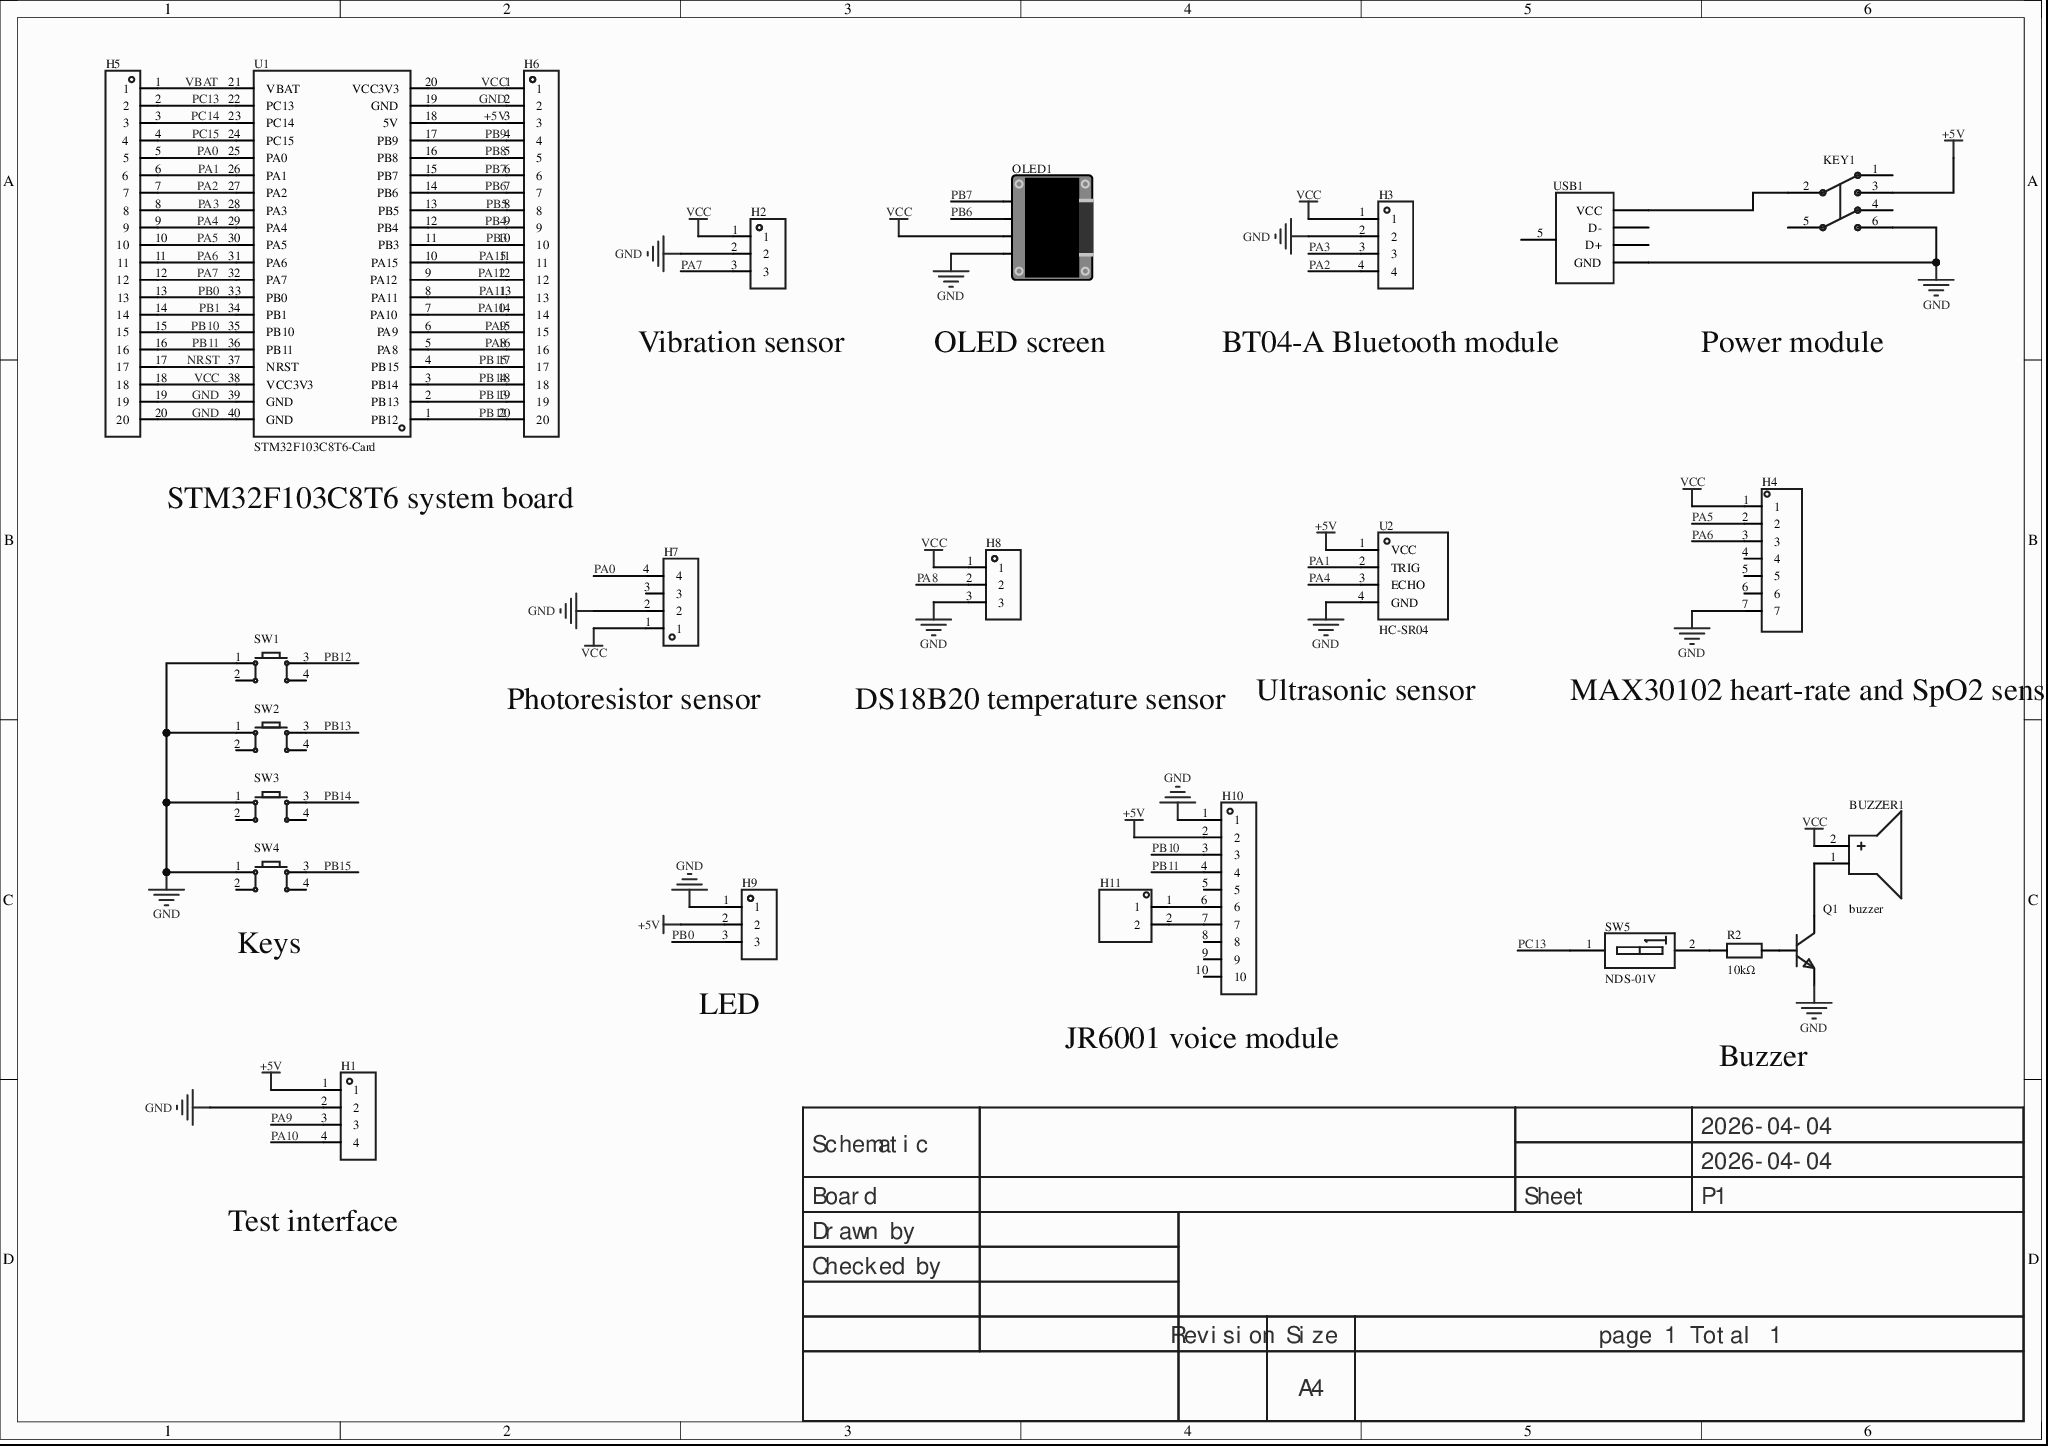
[diagram p0: MISC61230-3.schdoc]
# Altium project MISC61230-2.PrjPcb
1 sheet, 24 parts. Net scope: global (net labels, ports and power ports of the same name join across sheets).
Board file: MISC61230.pcbdoc

## Sheet MISC61230-3.schdoc
size 297 x 209 mm; Version: V1.0; @Project Name: MISC61230; @Page Count: 1; @Update Date: 2026-04-04; @Create Date: 2026-04-04; @Schematic Name: MISC61230; @Page No: 1; @Create Time: 18:58:15; @Update Time: 22:44:58; @Board Name: MISC61230

### Parts
BUZZER1  buzzer  [BUZ-TH_BD12.0-P6.00-D0.9-RD]
H1  (no value)  [HDR-TH_4P-P2.54-V-M]
H2  (no value)  [HDR-TH_3P-P2.54-V-F]
H3  (no value)  [HDR-TH_4P-P2.54-V-M]
H4  (no value)  [HDR-TH_7P-P2.54-V-F]
H5  (no value)  [HDR-TH_20P-P2.54-V-M-1]
H6  (no value)  [HDR-TH_20P-P2.54-V-M-1]
H7  (no value)  [HDR-TH_4P-P2.54-V-M]
H8  (no value)  [HDR-TH_3P-P2.54-V-F]
H9  (no value)  [HDR-TH_3P-P2.54-V-F]
H10  (no value)  [HDR-TH_10P-P2.54-V-F]
H11  (no value)  [HDR-TH_2P-P2.54-V-M-1]
KEY1  Non-latching switch 8.5×8.5, silent  [SW-TH_6P-L8.5-W8.5-P2.54]  (value not drawn)
OLED1  (no value)  [0.96OLED_4P]
Q1  (no value)  [S8050_TO_92]
R2  10kΩ  [Res_1/8W]
SW1  (no value)  [SW-TH_4P-L6.0-W6.0-P4.50-LS6.5]
SW2  (no value)  [SW-TH_4P-L6.0-W6.0-P4.50-LS6.5]
SW3  (no value)  [SW-TH_4P-L6.0-W6.0-P4.50-LS6.5]
SW4  (no value)  [SW-TH_4P-L6.0-W6.0-P4.50-LS6.5]
SW5  NDS-01V  [SW-TH_2P-L3.9-W9.9-P2.54-LS7.6]
U1  STM32F103C8T6-Card  [CONN-TH_L53.3-W22.9_STM32F103C8T6-CARD]
U2  HC-SR04  [TH_HC-SR04V]
USB1  (no value)  [USB_ Type-B]

### Nets
+5V: H1.1 H6.3 H9.2 H10.2 KEY1.3 U1.18(5V) U2.1(VCC)
GND: H1.2 H2.2 H3.2 H4.7 H5.19 H5.20 H6.2 H7.2 H8.3 H9.1 H10.1 KEY1.6 OLED1.1(GND) Q1.1(E) SW1.1 SW2.1 SW3.1 SW4.1 U1.19(GND) U1.39(GND) U1.40(GND) U2.4(GND) USB1.4(GND)
VCC: BUZZER1.2(+) H2.1 H3.1 H4.1 H5.18 H6.1 H7.1 H8.1 OLED1.2(VCC) U1.20(VCC3V3) U1.38(VCC3V3)
NRST: H5.17 U1.37(NRST)
PA0: H5.5 H7.4 U1.25(PA0)
PA1: H5.6 U1.26(PA1) U2.2(TRIG)
PA2: H3.4 H5.7 U1.27(PA2)
PA3: H3.3 H5.8 U1.28(PA3)
PA4: H5.9 U1.29(PA4) U2.3(ECHO)
PA5: H4.2 H5.10 U1.30(PA5)
PA6: H4.3 H5.11 U1.31(PA6)
PA7: H2.3 H5.12 U1.32(PA7)
PA8: H6.16 H8.2 U1.5(PA8)
PA9: H1.3 H6.15 U1.6(PA9)
PA10: H1.4 H6.14 U1.7(PA10)
PA11: H6.13 U1.8(PA11)
PA12: H6.12 U1.9(PA12)
PA15: H6.11 U1.10(PA15)
PB0: H5.13 H9.3 U1.33(PB0)
PB1: H5.14 U1.34(PB1)
PB3: H6.10 U1.11(PB3)
PB4: H6.9 U1.12(PB4)
PB5: H6.8 U1.13(PB5)
PB6: H6.7 OLED1.3(SCL) U1.14(PB6)
PB7: H6.6 OLED1.4(SDA) U1.15(PB7)
PB8: H6.5 U1.16(PB8)
PB9: H6.4 U1.17(PB9)
PB10: H5.15 H10.3 U1.35(PB10)
PB11: H5.16 H10.4 U1.36(PB11)
PB12: H6.20 SW1.3 U1.1(PB12)
PB13: H6.19 SW2.3 U1.2(PB13)
PB14: H6.18 SW3.3 U1.3(PB14)
PB15: H6.17 SW4.3 U1.4(PB15)
PC13: H5.2 SW5.1(A1) U1.22(PC13)
PC14: H5.3 U1.23(PC14)
PC15: H5.4 U1.24(PC15)
VBAT: H5.1 U1.21(VBAT)
NetBUZZER1_1: BUZZER1.1(-) Q1.3(C)
NetH10_6: H10.6 H11.1
NetH10_7: H10.7 H11.2
NetKEY1_2: KEY1.2 USB1.1(VCC)
NetQ1_2: Q1.2(B) R2.2
NetR2_1: R2.1 SW5.2(A2)

Not connected (* = marked no-connect by the designer): H4 4 5 6; H7 3; H10 5 8 9 10; KEY1 1 4 5; SW1 2 4; SW2 2 4; SW3 2 4; SW4 2 4; USB1 2(D-)* 3(D+)* 5(SH1)

### Notes on the sheet
- (near H2) Vibration sensor
- OLED screen
- BT04-A Bluetooth module
- Power module
- STM32F103C8T6 system board
- (near H7) Photoresistor sensor
- DS18B20 temperature sensor
- Ultrasonic sensor
- (near H4) MAX30102 heart-rate and SpO2 sensor
- (near SW4) Keys
- (near H9) LED
- (near H10) JR6001 voice module
- Buzzer
- (near H1) Test interface
- 2026-04-04
- Schematic
- Board
- Sheet
- P1
- Drawn by
- Checked by
- Revision
- Size
- A4
- page 1 Total 1

### Library data of the parts
BUZZER1 = buzzer: AddInBom: yes; ModelId: af17e4151ed84fc2a628230bf23763630819f05c4eef4c71ace90d822a990e87; ModelTransform: 472.44,472.176,0,270,0,0,0,0,-196.85; Symbol: BUZZER; Device: buzzer; LCSC Part Name: buzzer; SupplierPart: C9900014030; ManufacturerPart: buzzer; Supplier Footprint: buzzer; JLCPCB Part Class: Extended Part; Supplier: LCSC; ConvertToPcb: yes; FootprintName: BUZ-TH_BD12.0-P6.00-D0.9-RD; ModelName: BUZ-TH_BD12.0-P6.00-D0.9-RD
H1 = HDR-M_2.54_1x4P: Symbol: PZ254V-11-04P; ConvertToPcb: yes; ModelId: 112f4d05e8d64e99ab9a333894bea4f90819f05c4eef4c71ace90d822a990e87; ModelName: HDR-TH_4P-P2.54-M-LI-1X4P; ModelTransform: 399.999,104.7242,0,0,0,0,0,0,-118.11; Device: HDR-M_2.54_1x4P; AddInBom: yes; SupplierPart: C492403; Supplier Footprint: 插件; FootprintName: HDR-TH_4P-P2.54-V-M
H2 H8 H9 = HDR-F_2.54_1x3P: Symbol: PM254V-11-03-H85; 3D Model: f3b3cc5aae9641bf9e56fc160cef875b; 3D Model Transform: 299.9994,100,0,0,0,0,0,0,-118.11; ConvertToPcb: yes; ModelName: HDR2.54-F-LI-1X3P; Device: HDR-F_2.54_1x3P; Supplier Part: C541850; Supplier Footprint: 插件; AddInBom: yes; FootprintName: HDR-TH_3P-P2.54-V-F
H3 H7 = HDR-M_2.54_1x4P: Symbol: PZ254V-11-04P; 3D Model: 112f4d05e8d64e99ab9a333894bea4f90819f05c4eef4c71ace90d822a990e87; 3D Model Transform: 399.999,104.7242,0,0,0,0,0,0,-118.11; ConvertToPcb: yes; ModelName: HDR-TH_4P-P2.54-M-LI-1X4P; Device: HDR-M_2.54_1x4P; Supplier Part: C492403; Supplier Footprint: 插件; AddInBom: yes; FootprintName: HDR-TH_4P-P2.54-V-M
H4 = HDR-F_2.54_1x7P: Symbol: 220S-1*7P H=8.5MM Ytype Gold-plated; ConvertToPcb: yes; ModelId: 4c31987253bc43b9b52c17be2a6d3f910819f05c4eef4c71ace90d822a990e87; ModelName: HDR-TH_7P-P2.54-F-LI-1X7P; ModelTransform: 715.7466,94.488,0,0,0,0,0,0,-118.11; Device: HDR-F_2.54_1x7P; AddInBom: yes; SupplierPart: C124418; Supplier Footprint: 插件; FootprintName: HDR-TH_7P-P2.54-V-F
H5 H6 = HDR-M_2.54_1x20P: Pitch:2.54mm;total pins:20;rows:1;pin structure:-;row spacing:-;mounting type:through-hole;round/square pin:-;rated current:-;rated voltage:-;mating pin length:-;plastic height:-;contact material:brass;contact plating:-;colour:black;; Symbol: HDR_2.54-1x20P; ConvertToPcb: yes; ModelId: f68709be121d406db68b06f32a5953890819f05c4eef4c71ace90d822a990e87; ModelName: HDR-M-2.54_1x20; ModelTransform: 1999.996,100,0,0,0,0,0,0,-118.11; Device: HDR-M_2.54_1x20P; AddInBom: yes; SupplierPart: C50981; Supplier Footprint: 插件; FootprintName: HDR-TH_20P-P2.54-V-M-1
H10 = HDR-F_2.54_1x10P: Symbol: X5511FV-10-C70D30-1000; AddInBom: yes; ModelId: 08a5ee31ec6747838a696d2ac093ffa40819f05c4eef4c71ace90d822a990e87; ModelName: HDR-TH_10P-P2.54-F-LI-1X10P; ModelTransform: 1009.87987,100,0,0,0,0,0,0,-125.984; Device: HDR-F_2.54_1x10P; ConvertToPcb: yes; FootprintName: HDR-TH_10P-P2.54-V-F; SupplierPart: C2684744; Supplier Footprint: 插件
H11 = HDR-M_2.54_1x2P: Symbol: 210S-1*2P L=11.6MMGold-plated black; ConvertToPcb: yes; ModelId: 79b2e9f2d70a4d68a1b7098f27c6d4c50819f05c4eef4c71ace90d822a990e87; ModelName: HDR-M-2.54_1x2; ModelTransform: 200,100,0,0,0,0,0,0,-118.11; Device: HDR-M_2.54_1x2P; AddInBom: yes; SupplierPart: C124375; Supplier Footprint: 插件; FootprintName: HDR-TH_2P-P2.54-V-M-1
KEY1 = 无自锁开关 8.5×8.5 无声: 6-pin, 8.5×8.5; Symbol: No self-locking switch 8.5×8.5 silent; AddInBom: yes; ModelId: 4c72b3966b92446eb355e1bd0fb4f8800819f05c4eef4c71ace90d822a990e87; ModelTransform: 342.519,334.645,0,180,0,0,0,0,-137.795; Device: Non-latching switch 8.5×8.5, silent; LCSC Part Name: 无自锁开关 8.5×8.5  无声; SupplierPart: C26228; ManufacturerPart: 无自锁开关 8.5×8.5 无声; Supplier Footprint: 插件; JLCPCB Part Class: Extended Part; Supplier: LCSC; ConvertToPcb: yes; FootprintName: SW-TH_6P-L8.5-W8.5-P2.54; ModelName: SW-TH_6P-L8.5-W8.5-P2.54
OLED1 = 0.96OLED模块_4P: Symbol: 0.96OLED module_4P; ConvertToPcb: yes; ModelId: 79c000fdb68d45a296c2e9bedf4f9055; ModelTransform: 1393.69792,1318.895,0,0,0,0,0,-560.079,-137.795; Device: 0.96OLED module_4P; AddInBom: yes; FootprintName: 0.96OLED_4P; Supplier Footprint: 插件; ModelName: 0.96OLED_4P
Q1 = S8050_TO_NPN: ConvertToPcb: yes; ModelId: aafe8e06f2154e7c93506efd0d6632dd; ModelName: TO-92-3_L4.9-W3.7-P1.27-L; ModelTransform: 180.78,141.44,417.3,0,0,0,0,0,-200; Symbol: S8050_TO_NPN; Device: S8050_TO_NPN; AddInBom: yes; Supplier Footprint: TO-92; FootprintName: S8050_TO_92
R2 = Res_AXIAL-1/8W: Symbol: Resistor; ConvertToPcb: yes; ModelId: b2b5ae7ae4c642178fe0039925c86a3f; ModelName: RES-TH_BD1.8-L3.2-P7.20-D0.4; ModelTransform: 282.86,66.88,253.09,0,0,0,0,0,-191; Device: Res_AXIAL-1/8W; AddInBom: yes; Supplier Footprint: 轴向引线; Value: 10kΩ; FootprintName: Res_1/8W
SW1-SW4 = Key_TH_6x6x6: 触点电流:50mA;额定电压(DC):12V;绝缘电阻:100MΩ;电路结构:单刀单掷;安装方式:直插;按钮形状:圆形按钮;按钮/盖帽颜色:黑色;作用力:260gf@±30gf;工作温度:-25℃~+70℃;引脚样式:PC引脚;开关长度:6mm;开关宽度:6mm;开关高度:6mm;带支架:否;; Symbol: Tactile switch; AddInBom: yes; ModelId: 20eee248bc684ccd8cbdbb1d0d91ec6f0819f05c4eef4c71ace90d822a990e87; ModelName: SW-TH_4P-L6.0-W6.0-H5.0-LS6.5-P4.50; ModelTransform: 236.22,323.03,0,90,0,0,0,0,-137.795; Device: Key_TH_6x6x6; ConvertToPcb: yes; FootprintName: SW-TH_4P-L6.0-W6.0-P4.50-LS6.5; Supplier Footprint: 插件
SW5 = NDS-01V_C501305: Toggle lever, upright; AddInBom: yes; ModelId: a6fe51954c31461ebc9e88beb6e51f3d0819f05c4eef4c71ace90d822a990e87; ModelName: SW-TH_L4.0-W9.9-H5.4-P2.54-B; ModelTransform: 161.417,389.763,0,270,0,0,0,0,-125.984; Symbol: NDS-01V; Device: NDS-01V_C501305; LCSC Part Name: 拨码开关; SupplierPart: C501305; ManufacturerPart: NDS-01V; Supplier Footprint: DIP; JLCPCB Part Class: Extended Part; Supplier: LCSC; ConvertToPcb: yes; FootprintName: SW-TH_2P-L3.9-W9.9-P2.54-LS7.6
U1 = STM32F103C8T6-Card: AddInBom: yes; Symbol: STM32F103C8T6-CARD; Device: STM32F103C8T6-Card; LCSC Part Name: STM32F103C8T6-Card; SupplierPart: C9900077949; ManufacturerPart: STM32F103C8T6-Card; Supplier Footprint: 插件; Supplier: LCSC; ConvertToPcb: yes; FootprintName: CONN-TH_L53.3-W22.9_STM32F103C8T6-CARD
U2 = HC-SR04: Manufacturer: Universal Microelectronics; AddInBom: yes; Symbol: HC-SR04; Device: HC-SR04; LCSC Part Name: HC-SR04; SupplierPart: C19857336; ManufacturerPart: HC-SR04; Supplier Footprint: -; JLCPCB Part Class: Extended Part; Datasheet: https://example.com/datasheet/HC-SR04/21184790.html; Supplier: LCSC; ConvertToPcb: yes; FootprintName: TH_HC-SR04V
USB1 = USB_ Type-B: ConvertToPcb: yes; ModelId: bbf32347d5be4dcea8001c0804ac390e0819f05c4eef4c71ace90d822a990e87; ModelName: USB-B_TH_BF90; ModelTransform: 547.99,637.8,543.15,0,0,0,0,0,-125.98; Symbol: USB_ Type-B; Device: USB_ Type-B; AddInBom: yes; Supplier Footprint: 插件; FootprintName: USB_ Type-B